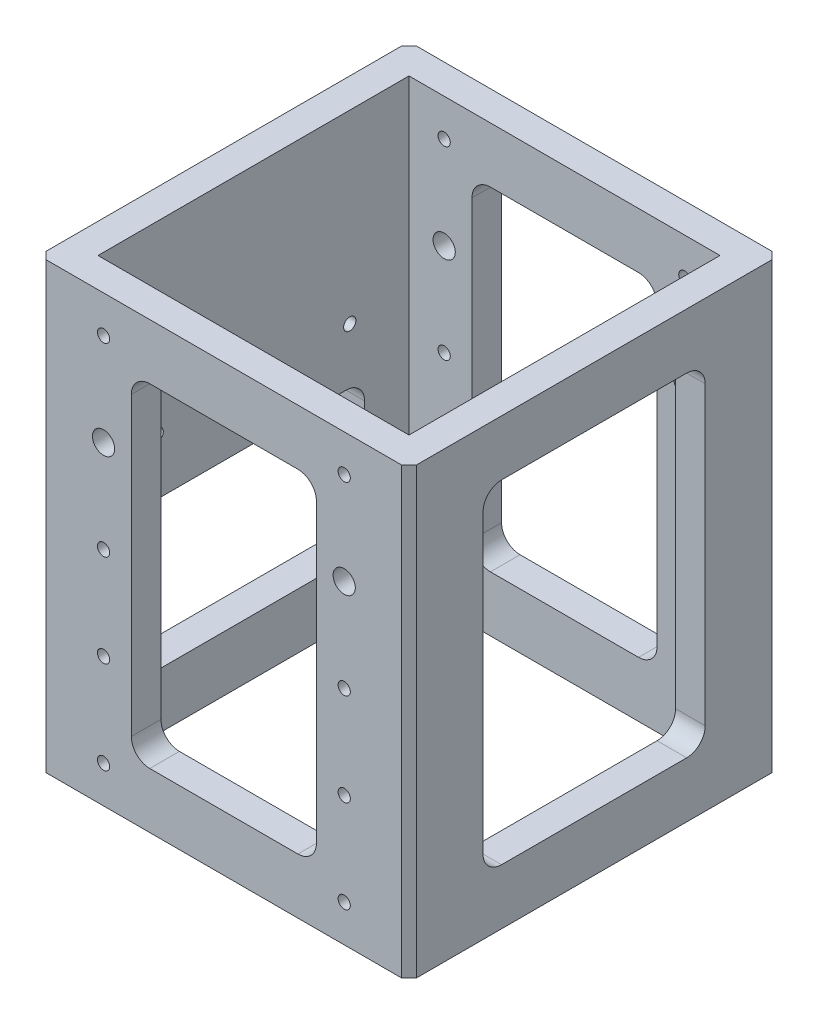
SolidWorks part; units mm, degrees
ref_plane "Front Plane" through (0, 0, 0) normal (0, 0, 1) x (1, 0, 0)
ref_plane "Top Plane" through (0, 0, 0) normal (0, 1, 0) x (1, 0, 0)
ref_plane "Right Plane" through (0, 0, 0) normal (1, 0, 0) x (0, 0, -1)
sketch "Sketch1" plane through (0, 0, 0) normal (0, 1, 0) x (1, 0, 0)
  line L0 (0, 0) -> (0, -50000) construction
  line L1 (-42, 50) -> (42, 50)
  line L2 (-42, 50) -> (-42, 42)
  line L3 (-42, -50) -> (42, -50)
  line L4 (42, 50) -> (42, 42)
  line L5 (-42, 50) -> (42, -50) construction
  line L6 (-42, -50) -> (42, 50) construction
  line L7 (-42, -42) -> (-42, -50)
  line L8 (-42, 42) -> (-3, 42)
  line L9 (42, -42) -> (3, -42)
  line L10 (-42, -42) -> (-3, -42)
  line L11 (-3, 42) -> (-3, -42)
  line L12 (3, 42) -> (3, -42)
  line L13 (42, 42) -> (3, 42)
  line L14 (42, -42) -> (42, -50)
  point P0 (0, 0)
  dimension "D1" = 8
  dimension "D2" = 8
  dimension "D3" = 3
  dimension "D4" = 100
  dimension "D5" = 84
extrude "Boss-Extrude1" add sketch "Sketch1" along normal blind 120
sketch "Sketch3" plane through (0, 120, 0) normal (0, 1, 0) x (1, 0, 0)
  line L0 (0, 50) -> (0, -49950) construction
  line L1 (-42, 50) -> (-50, 50)
  line L2 (-42, 50) -> (-42, -50)
  line L3 (-42, -50) -> (-50, -50)
  line L4 (-50, 50) -> (-50, -50)
  line L5 (42, 50) -> (-42, 50) construction
  line L6 (-42, -50) -> (42, -50) construction
  line L8 (50, 50) -> (50, -50)
  line L9 (42, -50) -> (50, -50)
  line L10 (42, 50) -> (42, -50)
  line L11 (42, 50) -> (50, 50)
  point P9 (0, 50)
  dimension "D1" = 8
extrude "Boss-Extrude2" add sketch "Sketch3" against normal up to surface (120 mm away) up to face at (0, 0, 0)
sketch "Sketch4" plane through (0, 120, 0) normal (0, 1, 0) x (1, 0, 0)
  line L1 (42, -42) -> (-42, -42)
  line L2 (42, -42) -> (42, 42)
  line L3 (42, 42) -> (-42, 42)
  line L4 (-42, -42) -> (-42, 42)
extrude "Cut-Extrude2" cut sketch "Sketch4" against normal through all
sketch "Sketch6" plane through (0, 0, 50) normal (0, 0, 1) x (1, 0, 0)
  line L0 (0, 120) -> (0, -49880) construction
  line L1 (-50, 120) -> (50, 120) construction
  line L2 (-40, 60) -> (49960, 60) construction
  line L3 (-50, 0) -> (-50, 120) construction
  line L4 (-32.5, 110) -> (-32.5, -49890) construction
  circle A0 centre (-32.5, 60) radius 1.0344
  circle A1 centre (32.5, 60) radius 1.0344
  circle A4 centre (-32.5, 110) radius 1
  circle A5 centre (32.5, 110) radius 1
  circle A6 centre (32.5, 10) radius 1
  circle A7 centre (-32.5, 10) radius 1
  point P16 (0, 120)
  point P21 (-50, 60)
  dimension "D3" = 2
  dimension "D1" = 65
  dimension "D2" = 100
extrude "Cut-Extrude4" cut sketch "Sketch6" against normal blind 7
hole_wizard "M4 Tapped Hole1" positions "3DSketch1" profile "Sketch7" tap size "M4" standard "Gb"
sketch3d "3DSketch1"
  line L0 (-32.5, 110, 43) -> (-32.5, 110, 50) construction
  line L1 (32.5, 110, 43) -> (32.5, 110, 50) construction
  line L2 (32.5, 10, 43) -> (32.5, 10, 50) construction
  line L3 (-32.5, 10, 43) -> (-32.5, 10, 50) construction
  line L4 (-32.5, 60, 43) -> (-32.5, 60, 50) construction
  line L5 (32.5, 60, 43) -> (32.5, 60, 50) construction
  point P21 (-32.5, 110, 50)
  point P25 (32.5, 110, 50)
  point P29 (32.5, 10, 50)
  point P33 (-32.5, 10, 50)
  point P38 (-32.5, 60, 50)
  point P42 (32.5, 60, 50)
sketch "Sketch7" plane through (-32.5, 110, 50) normal (1, 0, 0) x (0, -1, 0)
  line L0 (0, 0) -> (0, 11.0914)
  line L1 (0, 11.0914) -> (1.65, 10.1)
  line L2 (1.65, 10.1) -> (1.65, 0)
  line L5 (1.65, 0) -> (0, 0)
  line L10 (0, 11.0914) -> (-1.65, 10.1) construction
  line L11 (0, -6.35) -> (0, 107.95) construction
  dimension "螺纹孔钻头直径" = 3.3
  dimension "螺纹孔钻头深度" = 10.1
  dimension "导头角度" = 118
cosmetic thread "Cosmetic thread 1" parameters "D1"=6, "D2"=4
cosmetic thread "Cosmetic thread 2" parameters "D1"=6, "D2"=4
cosmetic thread "Cosmetic thread 3" parameters "D1"=6, "D2"=4
cosmetic thread "Cosmetic thread 4" parameters "D1"=6, "D2"=4
cosmetic thread "Cosmetic thread 5" parameters "D1"=6, "D2"=4
cosmetic thread "Cosmetic thread 6" parameters "D1"=6, "D2"=4
mirror "Mirror2" about plane through (0, 0, 0) normal (0, 0, 1) of "M4 Tapped Hole1"
hole_wizard "M4 Tapped Hole2" positions "Sketch9" profile "Sketch8" tap size "M4" standard "Gb"
sketch "Sketch9" plane through (-50, 0, 0) normal (-1, 0, 0) x (0, 0, 1)
  line L0 (0, 0) -> (0, 132.0443) construction
  line L2 (-50, 120) -> (50, 120) construction
  point P0 (-26, 70)
  point P2 (26, 70)
  point P15 (37, 70)
  dimension "D1" = 52
  dimension "D2" = 50
  dimension "D3" = 11
sketch "Sketch8" plane through (-50, 70, -26) normal (0, 1, 0) x (0, 0, 1)
  line L0 (0, 0) -> (0, 12.4914)
  line L1 (0, 12.4914) -> (1.65, 11.5)
  line L2 (1.65, 11.5) -> (1.65, 0)
  line L5 (1.65, 0) -> (0, 0)
  line L10 (0, 12.4914) -> (-1.65, 11.5) construction
  line L11 (0, -6.35) -> (0, 107.95) construction
  dimension "螺纹孔钻头直径" = 3.3
  dimension "螺纹孔钻头深度" = 11.5
  dimension "导头角度" = 118
cosmetic thread "Cosmetic thread 7" parameters "D1"=6, "D2"=4
cosmetic thread "Cosmetic thread 8" parameters "D1"=6, "D2"=4
cosmetic thread "Cosmetic thread 9" parameters "D1"=6, "D2"=4
hole_wizard "Ø6.0 (6) Diameter Hole1" positions "Sketch11" profile "Sketch10" hole size "Ø6.0" standard "Gb" end condition through all
sketch "Sketch11" plane through (0, 0, 50) normal (0, 0, 1) x (1, 0, 0)
  line L0 (0, 0) -> (0, 120) construction
  line L1 (-50, 120) -> (50, 120) construction
  point P0 (-32.5, 85)
  point P2 (32.5, 85)
  dimension "D1" = 65
  dimension "D2" = 35
sketch "Sketch10" plane through (-32.5, 85, 50) normal (1, 0, 0) x (0, -1, 0)
  line L0 (0, 0) -> (0, 100)
  line L1 (0, 100) -> (3, 100)
  line L2 (3, 100) -> (3, 0)
  line L5 (3, 0) -> (0, 0)
  line L11 (0, -6.35) -> (0, 107.95) construction
  dimension "通孔孔直径" = 6
  dimension "通孔孔深度" = 100
sketch "Sketch12" plane through (0, 0, 50) normal (0, 0, 1) x (1, 0, 0)
  line L0 (-50, 120) -> (50, 120) construction
  line L1 (-20, 105) -> (20, 105)
  line L2 (-25, 100) -> (-25, 20)
  line L3 (-20, 15) -> (20, 15)
  line L4 (25, 100) -> (25, 20)
  line L5 (-25, 105) -> (25, 15) construction
  line L6 (-25, 15) -> (25, 105) construction
  line L7 (-50, 0) -> (50, 0) construction
  arc A0 (-25, 20) -> (-20, 15) centre (-20, 20) ccw
  arc A1 (20, 15) -> (25, 20) centre (20, 20) ccw
  arc A2 (25, 100) -> (20, 105) centre (20, 100) ccw
  arc A3 (-20, 105) -> (-25, 100) centre (-20, 100) ccw
  point P0 (0, 60)
  dimension "D4" = 5
  dimension "D1" = 15
  dimension "D2" = 15
  dimension "D3" = 50
extrude "Cut-Extrude5" cut sketch "Sketch12" against normal through all
sketch "Sketch13" plane through (50, 0, 0) normal (1, 0, 0) x (0, 0, -1)
  line L0 (-50, 120) -> (50, 120) construction
  line L1 (-25, 105) -> (25, 105)
  line L2 (-30, 100) -> (-30, 20)
  line L3 (-25, 15) -> (25, 15)
  line L4 (30, 100) -> (30, 20)
  line L5 (-30, 105) -> (30, 15) construction
  line L6 (-30, 15) -> (30, 105) construction
  line L7 (50, 0) -> (-50, 0) construction
  arc A0 (-30, 20) -> (-25, 15) centre (-25, 20) ccw
  arc A1 (25, 15) -> (30, 20) centre (25, 20) ccw
  arc A2 (30, 100) -> (25, 105) centre (25, 100) ccw
  arc A3 (-25, 105) -> (-30, 100) centre (-25, 100) ccw
  point P0 (0, 60)
  dimension "D4" = 5
  dimension "D1" = 15
  dimension "D2" = 15
  dimension "D3" = 60
extrude "Cut-Extrude6" cut sketch "Sketch13" against normal up to next
sketch "Sketch14" plane through (-50, 0, 0) normal (-1, 0, 0) x (0, 0, 1)
  line L0 (50, 0) -> (-50, 0) construction
  line L1 (-25, 55) -> (25, 55)
  line L2 (-30, 50) -> (-30, 20)
  line L3 (-25, 15) -> (25, 15)
  line L4 (30, 50) -> (30, 20)
  line L5 (-30, 55) -> (30, 15) construction
  line L6 (-30, 15) -> (30, 55) construction
  arc A0 (-30, 20) -> (-25, 15) centre (-25, 20) ccw
  arc A1 (25, 15) -> (30, 20) centre (25, 20) ccw
  arc A2 (30, 50) -> (25, 55) centre (25, 50) ccw
  arc A3 (-25, 55) -> (-30, 50) centre (-25, 50) ccw
  point P0 (0, 35)
  dimension "D4" = 5
  dimension "D1" = 60
  dimension "D2" = 40
  dimension "D3" = 15
extrude "Cut-Extrude7" cut sketch "Sketch14" against normal up to next
hole_wizard "M4 Tapped Hole3" positions "Sketch16" profile "Sketch15" tap size "M4" standard "Gb"
sketch "Sketch16" plane through (0, 0, 50) normal (0, 0, 1) x (1, 0, 0)
  line L0 (0, 0) -> (0, 49.3465) construction
  line L2 (-50, 0) -> (50, 0) construction
  point P0 (-32.5, 35)
  point P2 (32.5, 35)
  dimension "D1" = 65
  dimension "D2" = 35
sketch "Sketch15" plane through (-32.5, 35, 50) normal (1, 0, 0) x (0, -1, 0)
  line L0 (0, 0) -> (0, 100)
  line L1 (0, 100) -> (1.65, 100)
  line L2 (1.65, 100) -> (1.65, 0)
  line L5 (1.65, 0) -> (0, 0)
  line L11 (0, -6.35) -> (0, 107.95) construction
  dimension "通孔螺纹孔钻头直径" = 3.3
  dimension "通孔螺纹孔钻头深度" = 100
cosmetic thread "Cosmetic thread 10" parameters "D2"=4
cosmetic thread "Cosmetic thread 11" parameters "D2"=4
mirror "Mirror3" about plane through (0, 0, 0) normal (0, 0, 1) of "M4 Tapped Hole3"
chamfer "Chamfer1" distance 2 angle 45 4 edges at (-50, 60, -50) (50, 60, -50) (50, 60, 50) (-50, 60, 50)
